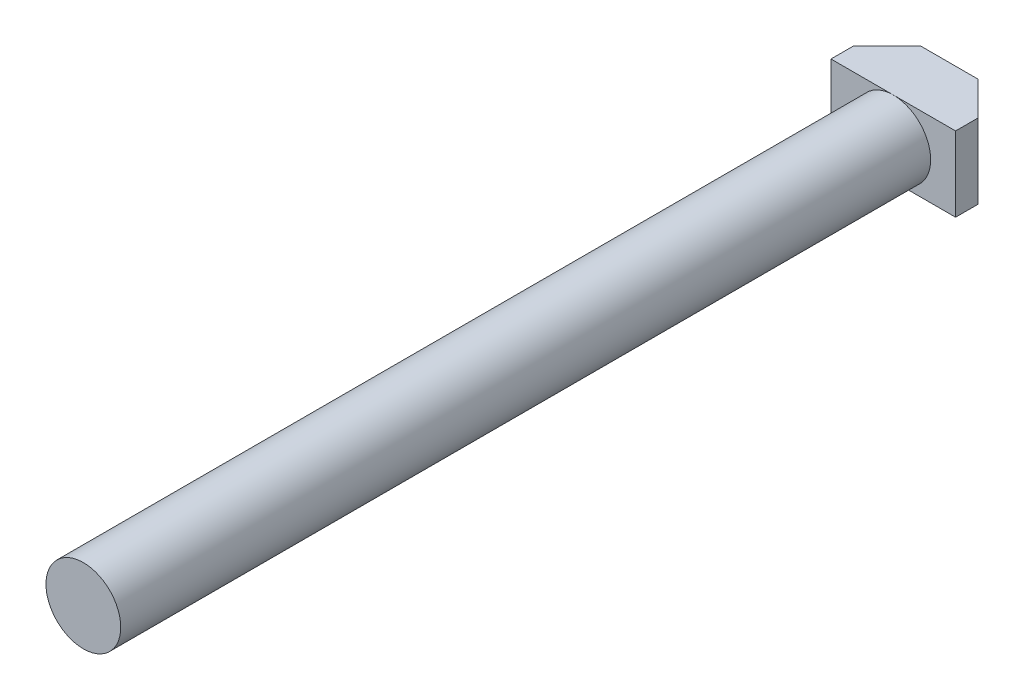
SolidWorks part; units mm, degrees
material "42CrMo"
ref_plane "Front Plane" through (0, 0, 0) normal (0, 0, 1) x (1, 0, 0)
ref_plane "Top Plane" through (0, 0, 0) normal (0, 1, 0) x (1, 0, 0)
ref_plane "Right Plane" through (0, 0, 0) normal (1, 0, 0) x (0, 0, -1)
sketch "Sketch1" plane through (0, 0, 0) normal (0, 1, 0) x (1, 0, 0)
  line L0 (-6.8797, 12.8683) -> (3.1203, 12.8683)
  line L1 (3.1203, 12.8683) -> (3.1203, 14.6683)
  line L2 (3.1203, 14.6683) -> (0.4203, 17.3683)
  line L3 (0.4203, 17.3683) -> (-4.1797, 17.3683)
  line L4 (-6.8797, 12.8683) -> (-6.8797, 14.6683)
  line L5 (-6.8797, 14.6683) -> (-4.1797, 17.3683)
  line L6 (-1.8797, 9.9248) -> (-1.8797, 19.0977) construction
  dimension "D1" = 10
  dimension "D2" = 135
  dimension "D3" = 1.8
  dimension "D4" = 4.5
extrude "Boss-Extrude1" add sketch "Sketch1" along normal blind 6
sketch "Sketch2" plane through (0, 0, -12.8683) normal (0, 0, 1) x (1, 0, 0)
  circle A0 centre (-1.8797, 3) radius 3
  dimension "D1" = 6
extrude "Boss-Extrude2" add sketch "Sketch2" along normal blind 65
cosmetic thread "Cosmetic Thread1" parameters "D1"=6.5, "D2"=4.917
ref_plane "Plane1" through (-1.8797, 0, 0) normal (1, 0, 0) x (0, 0, -1)
